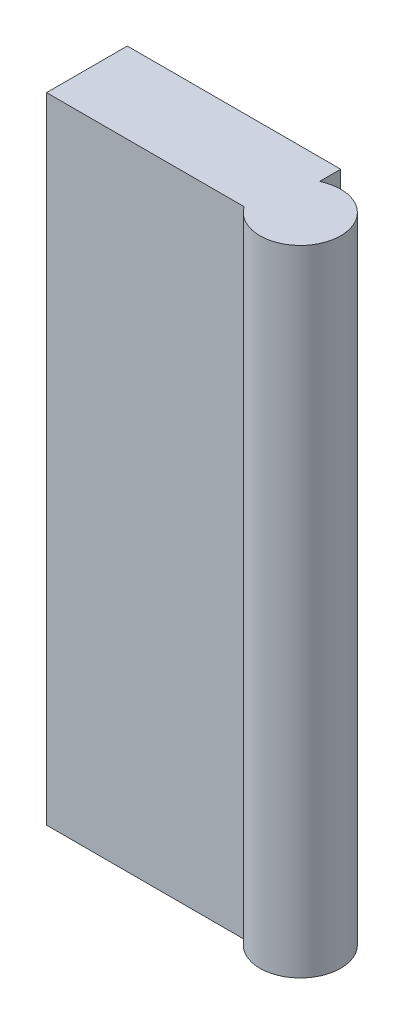
from build123d import *

# Parameters (mm, degrees)
SKETCH_1_W      = 18.5
SKETCH_1_H      = 55
EXTRUDE_1_DEPTH = 7
SKETCH_2_R      = 3.5
EXTRUDE_2_DEPTH = 55


with BuildPart() as part:
    # 草图1 → 凸台-拉伸1 (new body)
    with BuildSketch(Plane.XY):
        with Locations((9.25, 27.5)):
            Rectangle(SKETCH_1_W, SKETCH_1_H)
    extrude(amount=EXTRUDE_1_DEPTH)

    # 草图2 → 凸台-拉伸2 (add)
    with BuildSketch(Plane(origin=(0, 55, 0), x_dir=(1, 0, 0), z_dir=(0, 1, 0))):
        with Locations((20, -5)):
            Circle(SKETCH_2_R)
    extrude(amount=-EXTRUDE_2_DEPTH)


solid = part.part
